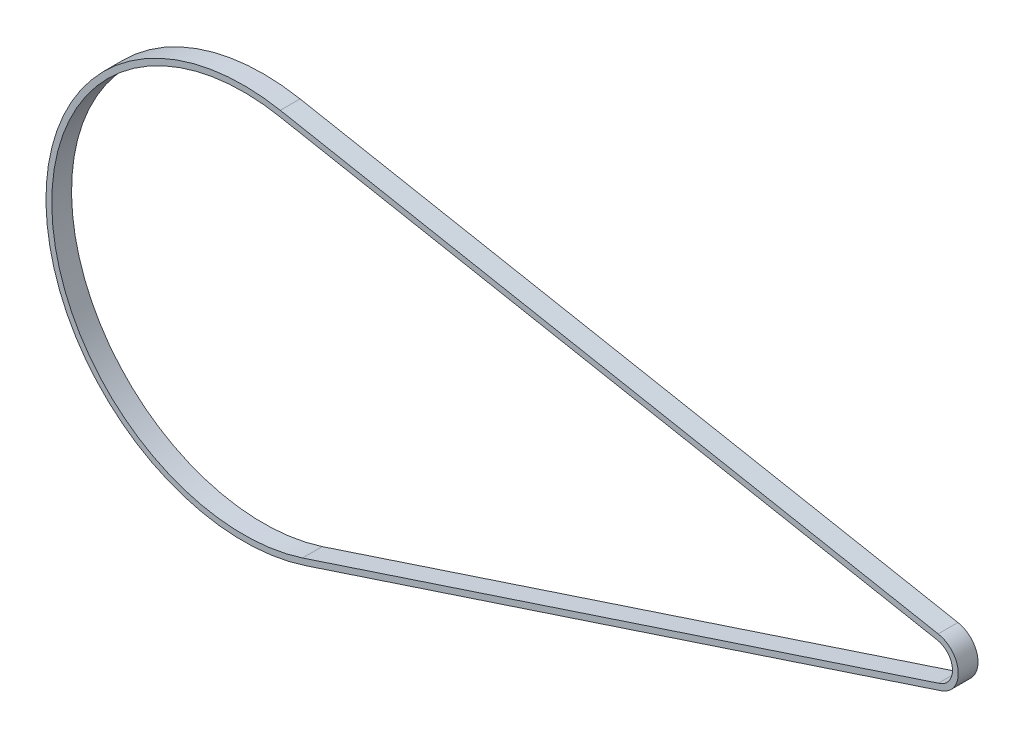
SolidWorks part; units mm, degrees
ref_plane "Front Plane" through (0, 0, 0) normal (0, 0, 1) x (1, 0, 0)
ref_plane "Top Plane" through (0, 0, 0) normal (0, 1, 0) x (1, 0, 0)
ref_plane "Right Plane" through (0, 0, 0) normal (1, 0, 0) x (0, 0, -1)
sketch "Sketch1" plane through (0, 0, 0) normal (0, 0, 1) x (1, 0, 0)
  line B0 (-803.4716, -72.5801) -> (-137.5148, -198.619)
  line B1 (-778.0713, -459.0448) -> (-134.3397, -246.9271)
  arc B2 (-803.4716, -72.5801) -> (-778.0713, -459.0448) centre (-840.6633, -269.0916) ccw
  arc B3 (-134.3397, -246.9271) -> (-137.5148, -198.619) centre (-142.1637, -223.1829) ccw
sketch_block_instance "Block 1-1-1"
sketch_block "Block 1-1"
ref_plane "Plane1" through (-803.4716, 0, 0) normal (1, 0, 0) x (0, 0, -1)
sketch "Sketch2" plane through (-803.4716, 0, 0) normal (1, 0, 0) x (0, 0, -1)
  line L0 (0, 0) -> (0, -99.4726) construction
  line L1 (-10, -72.5801) -> (10, -72.5801)
  line L2 (-10, -72.5801) -> (-10, -78.5801)
  line L3 (-10, -78.5801) -> (10, -78.5801)
  line L4 (10, -72.5801) -> (10, -78.5801)
  line L5 (0, -72.5801) -> (44.4298, -72.5801) construction
  dimension "D1" = 6
  dimension "D2" = 20
sweep "Sweep1" add profiles "Sketch2" path "Sketch1"
